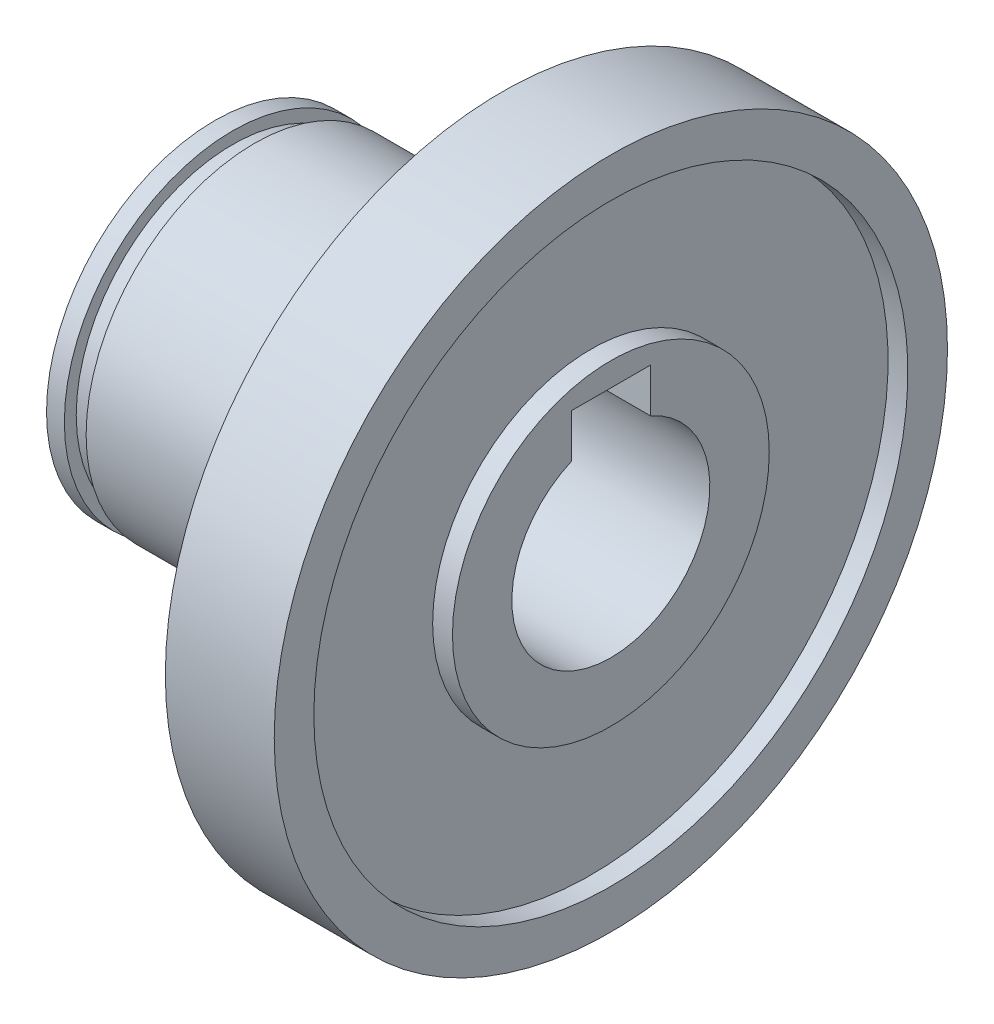
from build123d import *

# Parameters (mm, degrees)
SKETCH_2_W          = 4
SKETCH_2_H          = 6.8
CUT_EXTRUDE_1_DEPTH = 32.272991542


with BuildPart() as part:
    # 草图1 → 旋转1 (revolve)
    with BuildSketch(Plane.XY, mode=Mode.PRIVATE) as revolve_1_sk:
        Polygon((0, 5), (20, 5), (20, 8), (19, 8), (19, 15), (20, 15), (20, 17), (14.5, 17), (14.5, 8.5), (2, 8.5), (2, 7.9), (0.9, 7.9), (0.9, 8.5), (0, 8.5), align=None)
    revolve(revolve_1_sk.sketch.rotate(Axis((0, 0, 0), (1, 0, 0)), 90), axis=Axis((0, 0, 0), (1, 0, 0)))

    # 草图2 → 切除-拉伸1 (cut, through all)
    with BuildSketch(Plane(origin=(20, 0, 0), x_dir=(0, 0, -1), z_dir=(1, 0, 0))):
        with Locations((0, 3.4)):
            Rectangle(SKETCH_2_W, SKETCH_2_H)
    extrude(amount=-CUT_EXTRUDE_1_DEPTH, mode=Mode.SUBTRACT)


solid = part.part
